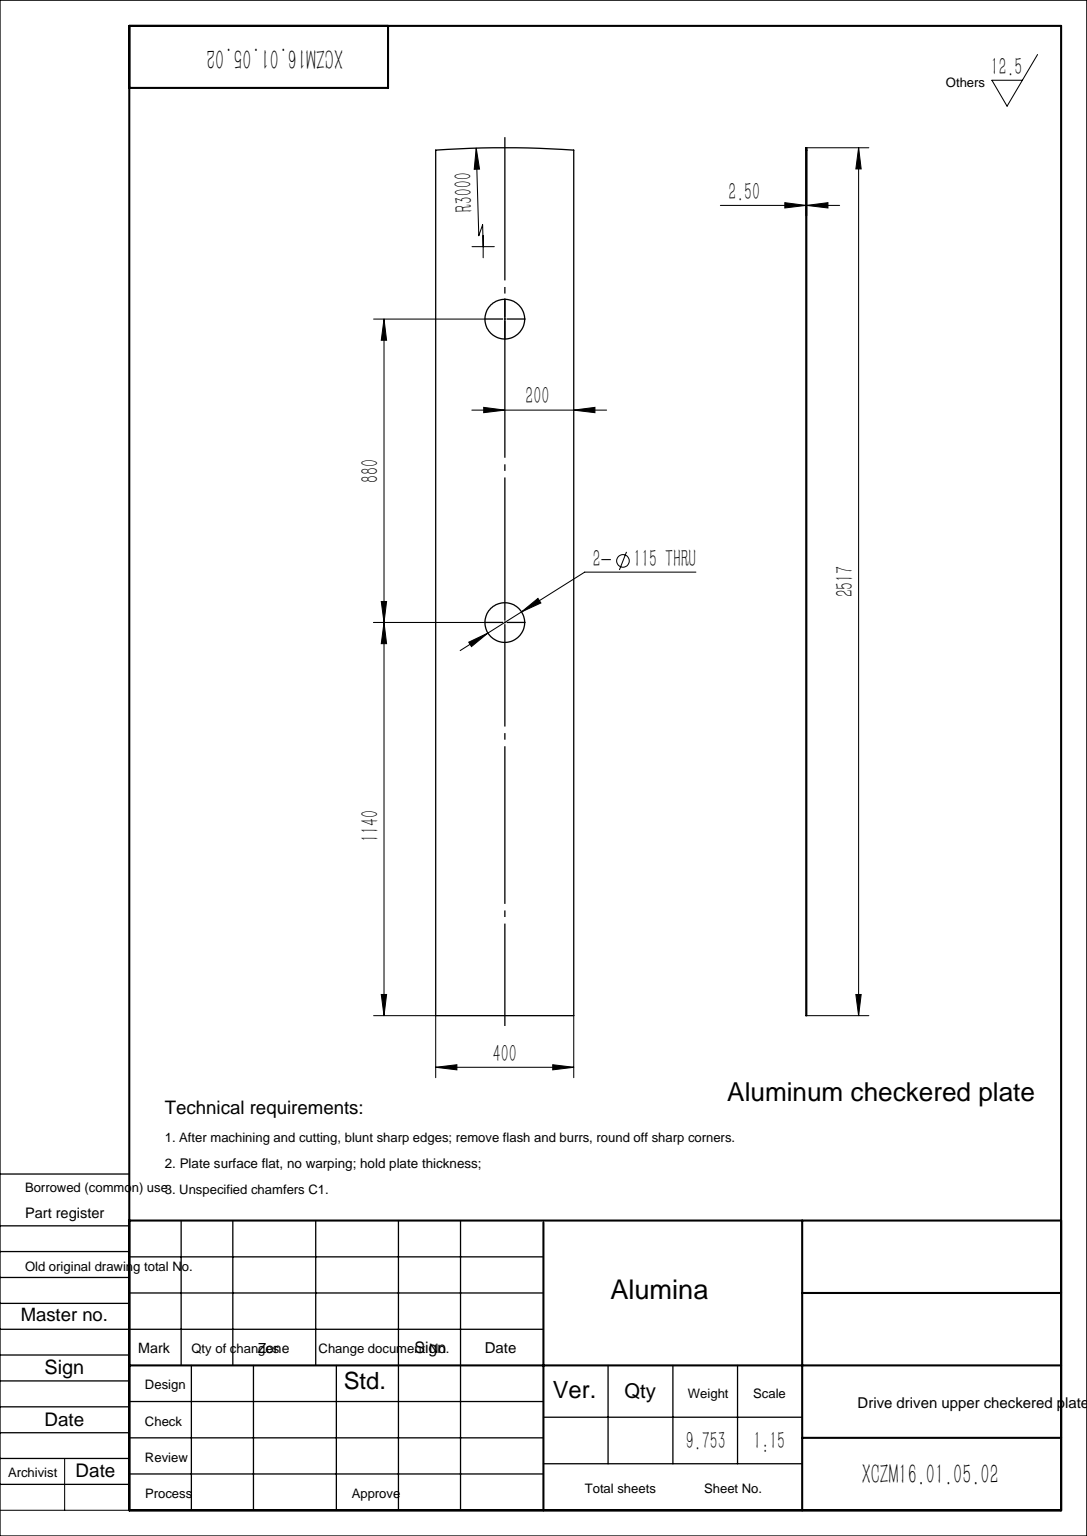
from build123d import *

# Parameters (mm, degrees)
SKETCH1_R           = 57.5
BOSS_EXTRUDE1_DEPTH = 2.5


with BuildPart() as part:
    # Sketch1 → Boss-Extrude1 (new body)
    with BuildSketch(Plane.XY):
        with BuildLine():
            Line((-200, 0), (200, 0))
            Line((200, 0), (200, 2510.325909419))
            ThreePointArc((200, 2510.325909419), (0, 2517), (-200, 2510.325909419))
            Line((-200, 2510.325909419), (-200, 0))
        make_face()
        with Locations((0, 2020)):
            Circle(SKETCH1_R, mode=Mode.SUBTRACT)
        with Locations((0, 1140)):
            Circle(SKETCH1_R, mode=Mode.SUBTRACT)
    extrude(amount=BOSS_EXTRUDE1_DEPTH)


solid = part.part
